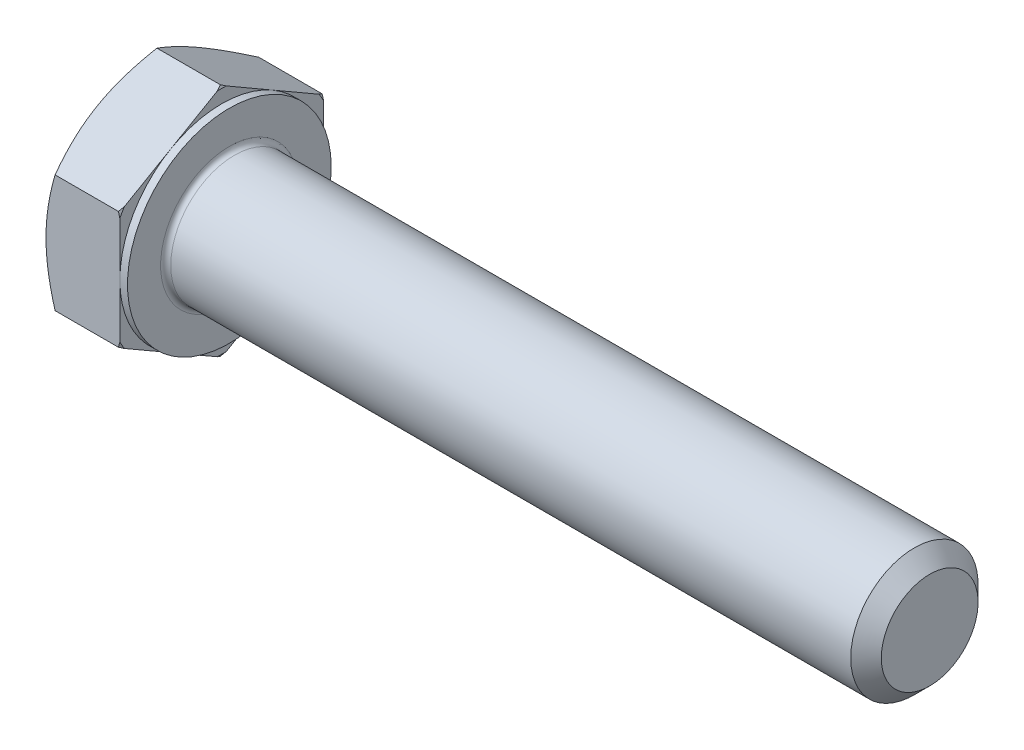
SolidWorks part; units mm, degrees
extrude "基体-拉伸" add sketch "草图1" along normal blind 6.4
sketch "草图1" plane through (0, 0, 0) normal (1, 0, 0) x (0, 0, -1)
  line L0 (8, 4.6188) -> (8, -4.6188)
  line L1 (-8, 4.6188) -> (-8, -4.6188)
  line L2 (8, -4.6188) -> (0, -9.2376)
  line L3 (0, -9.2376) -> (-8, -4.6188)
  line L4 (8, 4.6188) -> (0, 9.2376)
  line L5 (0, 9.2376) -> (-8, 4.6188)
revolve "切除-旋转1" cut sketch "草图3" angle 360 about L6
sketch "草图3" plane through (0, 0, 0) normal (0, 0, 1) x (1, 0, 0)
  line L0 (0, 8) -> (3.6013, 14.2376)
  line L1 (0, 9.2376) -> (0, 4.6188) construction
  line L2 (3.6013, 14.2376) -> (3.6013, 19.2376)
  line L3 (3.6013, 19.2376) -> (-10, 19.2376)
  line L4 (-10, 19.2376) -> (-10, 8)
  line L5 (-10, 8) -> (0, 8)
  line L6 (0, 0) -> (99.06, 0) construction
  line L7 (6.4, 9.2376) -> (0, 9.2376) construction
material "3.6级"
ref_plane "前视" through (0, 0, 0) normal (0, 0, 1) x (1, 0, 0)
ref_plane "上视" through (0, 0, 0) normal (0, 1, 0) x (1, 0, 0)
ref_plane "右视" through (0, 0, 0) normal (1, 0, 0) x (0, 0, -1)
sketch "草图2" plane through (0, 0, 0) normal (0, 0, 1) x (1, 0, 0)
  line L0 (0, 4.6188) -> (0, -4.6188) construction
  line L1 (0, 0) -> (61.4, 0)
  line L2 (0, 0) -> (0, 5)
  line L3 (0, 5) -> (27.8072, 5)
  line L4 (61.4, 0) -> (61.4, 3.701)
  line L5 (6.4, 9.2376) -> (6.4, 4.6188) construction
  line L7 (0, 0) -> (96.52, 0) construction
  line L8 (61.4, -3.701) -> (27.8072, -5) construction
  line L9 (0, -5) -> (27.8072, -5) construction
  line L10 (7.9, 15.24) -> (7.9, -1.27) construction
  line L11 (35.4, 15.24) -> (35.4, -1.27) construction
  line L12 (6.4, 4.6188) -> (6.4, -4.6188) construction
  line L13 (27.8072, 5) -> (61.4, 5)
  line L14 (61.4, 5) -> (61.4, 3.701)
revolve "凸台-旋转1" add sketch "草图2" angle 360 about L7
cosmetic thread "螺旋线1" parameters "Thread_length"=26, "Thread_minor"=7.402
sketch "草图5" plane through (0, 0, 0) normal (0, 0, 1) x (1, 0, 0)
  line L0 (6.4, 8) -> (2.7987, 14.2376)
  line L1 (6.4, 9.2376) -> (6.4, 4.6188) construction
  line L2 (2.7987, 14.2376) -> (2.7987, 19.2376)
  line L3 (2.7987, 19.2376) -> (12.7987, 19.2376)
  line L4 (12.7987, 19.2376) -> (12.7987, 8)
  line L5 (12.7987, 8) -> (6.4, 8)
  line L7 (6.4, 9.2376) -> (0.7145, 9.2376) construction
  line L8 (0, 0) -> (99.06, 0) construction
  line L9 (0, 0) -> (99.06, 0) construction
revolve "切除-旋转2" cut sketch "草图5" angle 360 about L8
sketch "草图4" plane through (0, 0, 0) normal (0, 0, 1) x (1, 0, 0)
  line L1 (6.4, 9.2376) -> (6.4, 4.6188) construction
  line L2 (6.4, 8) -> (5.8, 8)
  line L3 (6.4, 8) -> (6.4, 19.2376)
  line L4 (6.4, 19.2376) -> (5.8, 19.2376)
  line L5 (0, 0) -> (95.25, 0) construction
  line L6 (0, 0) -> (96.52, 0) construction
  line L7 (5.8, 8) -> (5.8, 19.2376)
  line L8 (5.6855, 9.2376) -> (0.7145, 9.2376) construction
revolve "切除-旋转3" cut sketch "草图4" angle 360 about L5
chamfer "倒角" distance 1.2 angle 45 1 edges at (61.4, 0, 5)
fillet "圆角" radius 0.4 1 edges at (6.4, 0, -5)
sketch "草图6" plane through (0, 0, 0) normal (0, 0, 1) x (1, 0, 0)
  line L0 (35.4, -3.701) -> (34.65, -5)
  line L1 (35.4, -3.701) -> (36.15, -5)
  line L2 (36.15, -5) -> (36.15, -6.25)
  line L3 (-3.175, 0) -> (5.1513, 0) construction
  line L5 (36.15, -6.25) -> (34.65, -6.25)
  line L6 (34.65, -6.25) -> (34.65, -5)
revolve "切除-旋转4" [suppressed] cut sketch "草图6" angle 360 about L3
pattern_linear "阵列(线性)1" [suppressed]
equation "\"D3@草图1\" = \"s@草图1\" / 2"
equation "\"D4@草图1\" = \"D3@草图1\""
equation "\"D5@草图1\" = \"D4@草图1\""
equation "\"Thread_minor@螺旋线1\" = \"Minor_dia@草图2\""
equation "\"D1@草图3\" = \"s@草图1\" / 2"
equation "\"D1@草图5\" = \"s@草图1\" / 2"
equation "\"Head_ch_ang@草图5\" = \"Head_ch_ang@草图3\""
equation "\"D1@草图4\" = \"s@草图1\""
equation "\"Thread_length@螺旋线1\" = ((sgn( (\"l@草图2\" - \"p@草图2\" ) - \"h@草图2\" )-1)*( (\"l@草图2\" - \"p@草图2\" ) - \"h@草图2\" ))/-2+ \"h@草图2\""
equation "\"Thread_minor@草图6\" = \"Minor_dia@草图2\""
equation "\"Diameter@草图6\" = \"m@草图2\""
equation "\"Overcut@草图6\" = \"m@草图2\" * 1.25"
equation "\"Start@草图6\" = \"k@基体-拉伸\" + \"l@草图2\" - \"Thread_length@螺旋线1\"  '---Non-countersunk---"
equation "\"Num_threads@阵列(线性)1\" = int( \"Thread_length@螺旋线1\" / \"p@草图2\" + 0.999 )  + 1"
equation "\"Advance@阵列(线性)1\" = \"Thread_length@螺旋线1\" /  (\"Num_threads@阵列(线性)1\" - 1) 'relax it"
equation "\"Num_threads@阵列(线性)1\" = \"Num_threads@阵列(线性)1\" - sgn( \"Num_threads@阵列(线性)1\" - 1) '---chamfered tips only---"
equation "\"Minor_dia@草图2\" = \"m@草图2\"-\"p@草图2\" * 1.732"
equation "\"D1@倒角\" = \"p@草图2\"*0.8"
